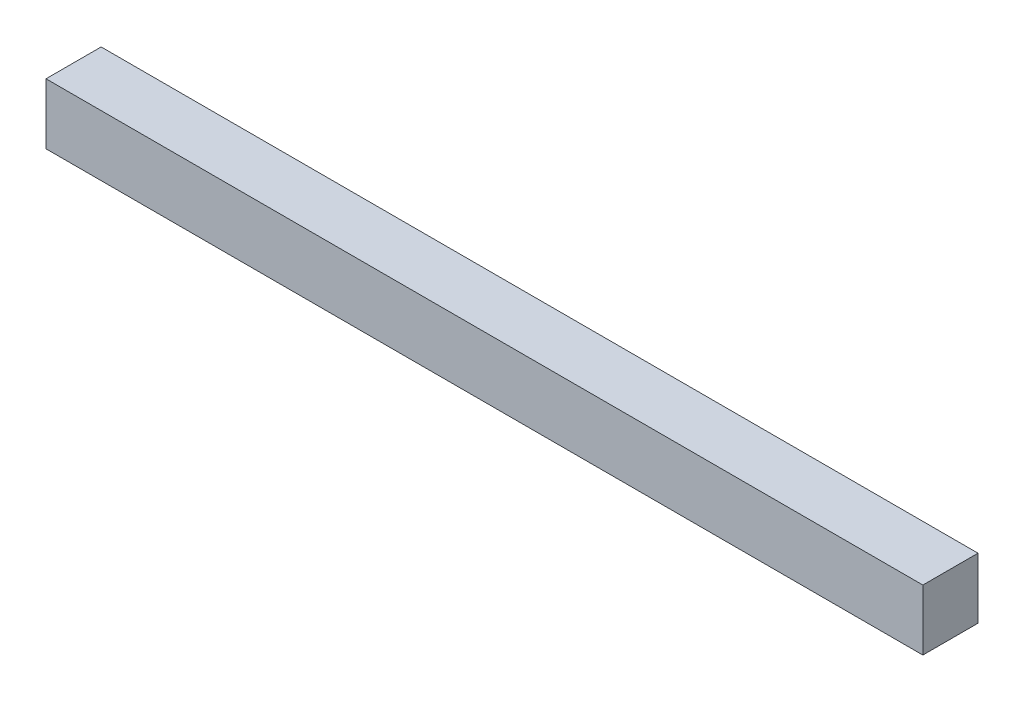
from build123d import *

# Parameters (mm, degrees)
SKETCH1_W           = 318
SKETCH1_H           = 22
BOSS_EXTRUDE1_DEPTH = 20


with BuildPart() as part:
    # Sketch1 → Boss-Extrude1 (new body)
    with BuildSketch(Plane.XY):
        with Locations((159, 11)):
            Rectangle(SKETCH1_W, SKETCH1_H)
    extrude(amount=BOSS_EXTRUDE1_DEPTH)


solid = part.part
